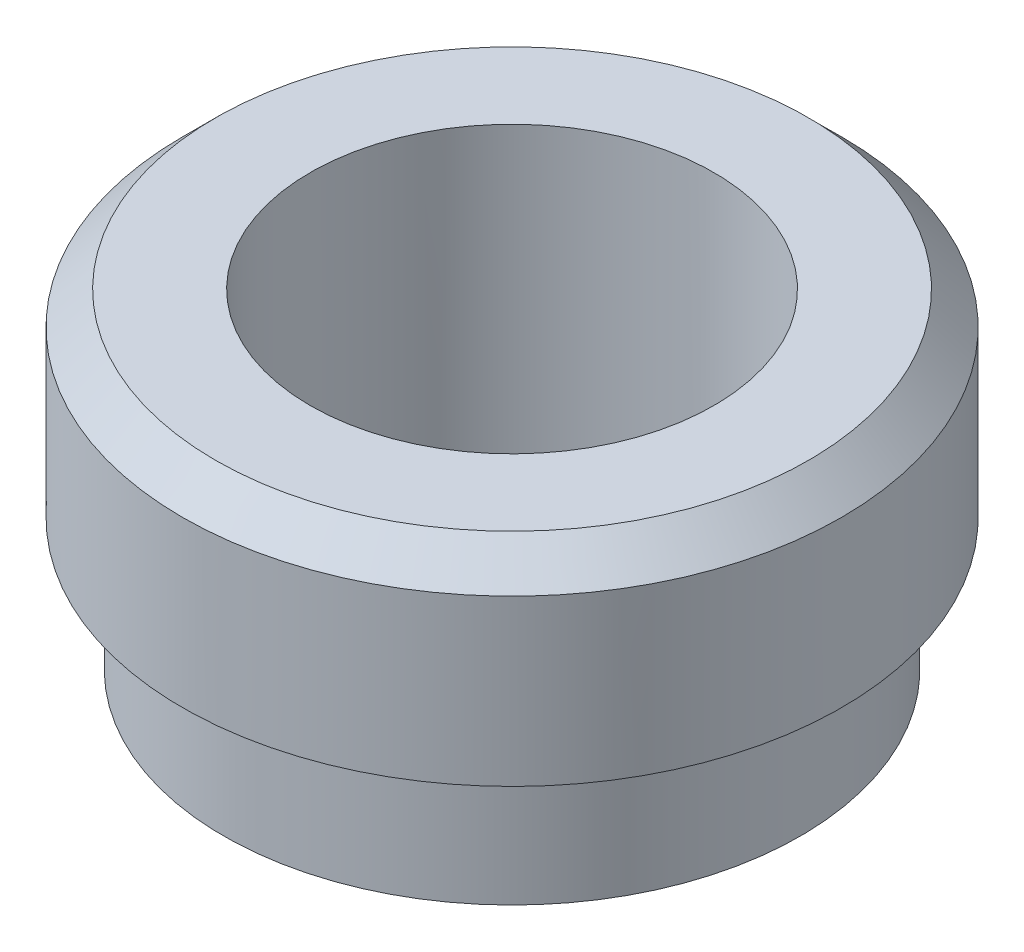
SolidWorks part; units mm, degrees
material "Q235"
ref_plane "Front Plane" through (0, 0, 0) normal (0, 0, 1) x (1, 0, 0)
ref_plane "Top Plane" through (0, 0, 0) normal (0, 1, 0) x (1, 0, 0)
ref_plane "Right Plane" through (0, 0, 0) normal (1, 0, 0) x (0, 0, -1)
sketch "Sketch1" plane through (0, 0, 0) normal (0, 0, 1) x (1, 0, 0)
  line L0 (0, 0) -> (20, 0)
  line L1 (20, 0) -> (20, -12)
  line L2 (20, -12) -> (17.5, -12)
  line L3 (17.5, -12) -> (17.5, -20)
  line L4 (17.5, -20) -> (0, -20)
  line L5 (0, -20) -> (0, 0)
  dimension "D1" = 17.5
  dimension "D2" = 20
  dimension "D3" = 8
  dimension "D4" = 12
revolve "Revolve1" add sketch "Sketch1" angle 360 about L5
hole_wizard "G3/4 Tapped Hole1" positions "Sketch2" profile "Sketch3" tap size "G3/4" standard "GB"
sketch "Sketch2" plane through (0, 0, 0) normal (0, 1, 0) x (1, 0, 0)
  point P0 (0, 0)
sketch "Sketch3" plane through (0, 0, 0) normal (1, 0, 0) x (0, 0, 1)
  line L0 (0, 0) -> (0, 65.6805)
  line L1 (0, 65.6805) -> (12.25, 58.32)
  line L2 (12.25, 58.32) -> (12.25, 0)
  line L5 (12.25, 0) -> (0, 0)
  line L10 (0, 65.6805) -> (-12.25, 58.32) construction
  line L11 (0, -6.35) -> (0, 107.95) construction
  dimension "螺纹孔钻头直径" = 24.5
  dimension "螺纹孔钻头深度" = 58.32
  dimension "导头角度" = 118
cosmetic thread "Hole cosmetic thread1" parameters "D1"=20, "D2"=26.441
chamfer "Chamfer1" distance 2 angle 45 1 edges at (0, 0, -20)
